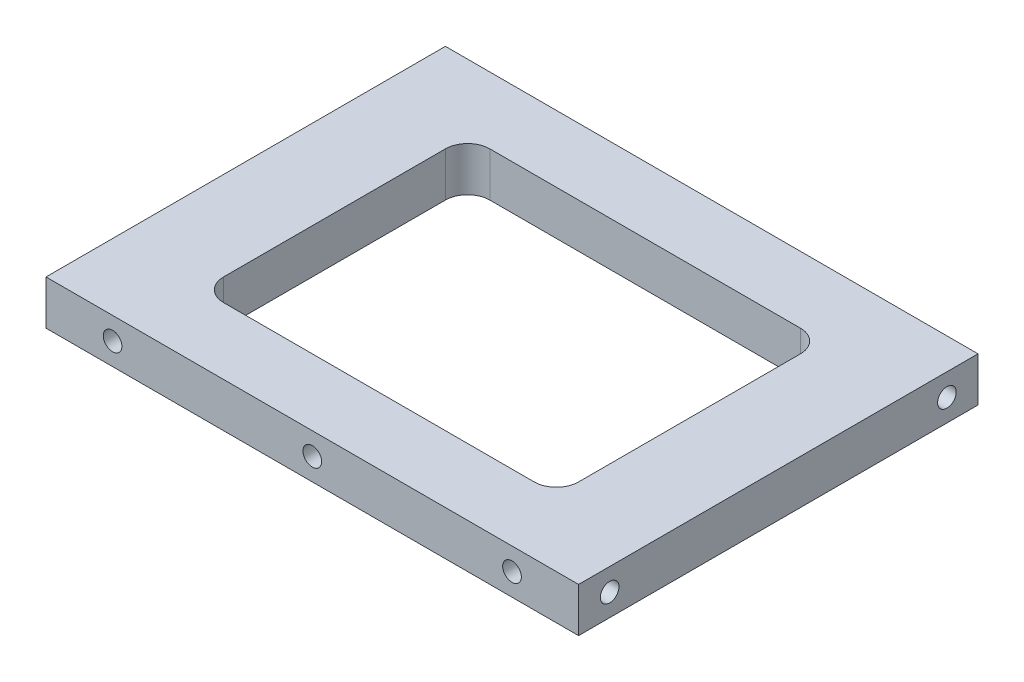
from build123d import *

# Parameters (mm, degrees)
SKETCH1_W                  = 120
SKETCH1_H                  = 90
BOSS_EXTRUDE1_DEPTH        = 10
SKETCH2_R                  = 0.808722662
CUT_EXTRUDE1_DEPTH         = 8
M5_TAPPED_HOLE1_AT_2_COUNT = 2
M5_TAPPED_HOLE1_AT_2_PITCH = 76
SKETCH4_R                  = 1.068128835
SKETCH4_R_2                = 0.756333918
SKETCH4_R_3                = 1.055288756
CUT_EXTRUDE2_DEPTH         = 6.5
M5_TAPPED_HOLE2_D          = 4.2
M5_TAPPED_HOLE2_DEPTH      = 12.4
M5_TAPPED_HOLE2_TIP        = 1.2618073
CUT_EXTRUDE3_DEPTH         = 76.663729812


with BuildPart() as part:
    # Sketch1 → Boss-Extrude1 (new body)
    with BuildSketch(Plane(origin=(0, 0, 0), x_dir=(1, 0, 0), z_dir=(0, 1, 0))):
        Rectangle(SKETCH1_W, SKETCH1_H)
    extrude(amount=BOSS_EXTRUDE1_DEPTH)

    # Sketch2 → Cut-Extrude1 (cut)
    with BuildSketch(Plane.ZY.offset(60)):
        with Locations(Location((-38, 5, 0), (0, 0, 180))):
            Circle(SKETCH2_R)
        with Locations((38, 5)):
            Circle(SKETCH2_R)
    extrude(amount=-CUT_EXTRUDE1_DEPTH, mode=Mode.SUBTRACT)

    # Sketch3 → M5 Tapped Hole1 (revolve, cut)
    with BuildSketch(Plane(origin=(-60, 5, 38), x_dir=(0, 0, 1), z_dir=(0, 1, 0))):
        Polygon((0, 0), (0, 13.6618073), (2.1, 12.4), (2.1, 0), align=None)
    m5_tapped_hole1 = revolve(axis=Axis((-66.35, 5, 38), (1, 0, 0)), mode=Mode.SUBTRACT)

    # M5 Tapped Hole1 at 2: M5 Tapped Hole1 ×2
    with Locations(*[(0, 0, -i * M5_TAPPED_HOLE1_AT_2_PITCH) for i in range(1, M5_TAPPED_HOLE1_AT_2_COUNT)]):
        add(m5_tapped_hole1, mode=Mode.SUBTRACT)

    # Mirror1: M5 Tapped Hole1 across plane
    add(m5_tapped_hole1.mirror(Plane(origin=(0, 0, 0), x_dir=(0, 0, 1), z_dir=(1, 0, 0))), mode=Mode.SUBTRACT)

    # Mirror1 copy 1 sketch → Mirror1 copy 1 (revolve, cut)
    with BuildSketch(Plane(origin=(60, 5, -38), x_dir=(0, 0, 1), z_dir=(0, 1, 0))):
        Polygon((0, 0), (0, -13.6618073), (2.1, -12.4), (2.1, 0), align=None)
    revolve(axis=Axis((66.35, 5, -38), (1, 0, 0)), mode=Mode.SUBTRACT)

    # Sketch4 → Cut-Extrude2 (cut)
    with BuildSketch(Plane.XY.offset(45)):
        with Locations((45, 5)):
            Circle(SKETCH4_R)
        with Locations((0, 5)):
            Circle(SKETCH4_R_2)
        with Locations((-45, 5)):
            Circle(SKETCH4_R_3)
    extrude(amount=-CUT_EXTRUDE2_DEPTH, mode=Mode.SUBTRACT)

    # M5 Tapped Hole2
    with Locations(Plane(origin=(-45, 5, 45), x_dir=(1, 0, 0), z_dir=(0, 0, 1))):
        with Locations((0, 0), (45, 0), (90, 0)):
            Hole(M5_TAPPED_HOLE2_D / 2, depth=M5_TAPPED_HOLE2_DEPTH)
            with Locations((0, 0, -(M5_TAPPED_HOLE2_DEPTH + M5_TAPPED_HOLE2_TIP / 2))):  # 118° drill point
                Cone(0, M5_TAPPED_HOLE2_D / 2, M5_TAPPED_HOLE2_TIP, mode=Mode.SUBTRACT)

    # Sketch6 → Cut-Extrude3 (cut, through all)
    with BuildSketch(Plane.XZ):
        with BuildLine():
            Line((-35, 30), (35, 30))
            ThreePointArc((35, 30), (38.535533906, 28.535533906), (40, 25))
            Line((40, 25), (40, -25))
            ThreePointArc((40, -25), (38.535533906, -28.535533906), (35, -30))
            Line((35, -30), (-35, -30))
            ThreePointArc((-35, -30), (-38.535533906, -28.535533906), (-40, -25))
            Line((-40, -25), (-40, 25))
            ThreePointArc((-40, 25), (-38.535533906, 28.535533906), (-35, 30))
        make_face()
    extrude(amount=-CUT_EXTRUDE3_DEPTH, mode=Mode.SUBTRACT)


solid = part.part
